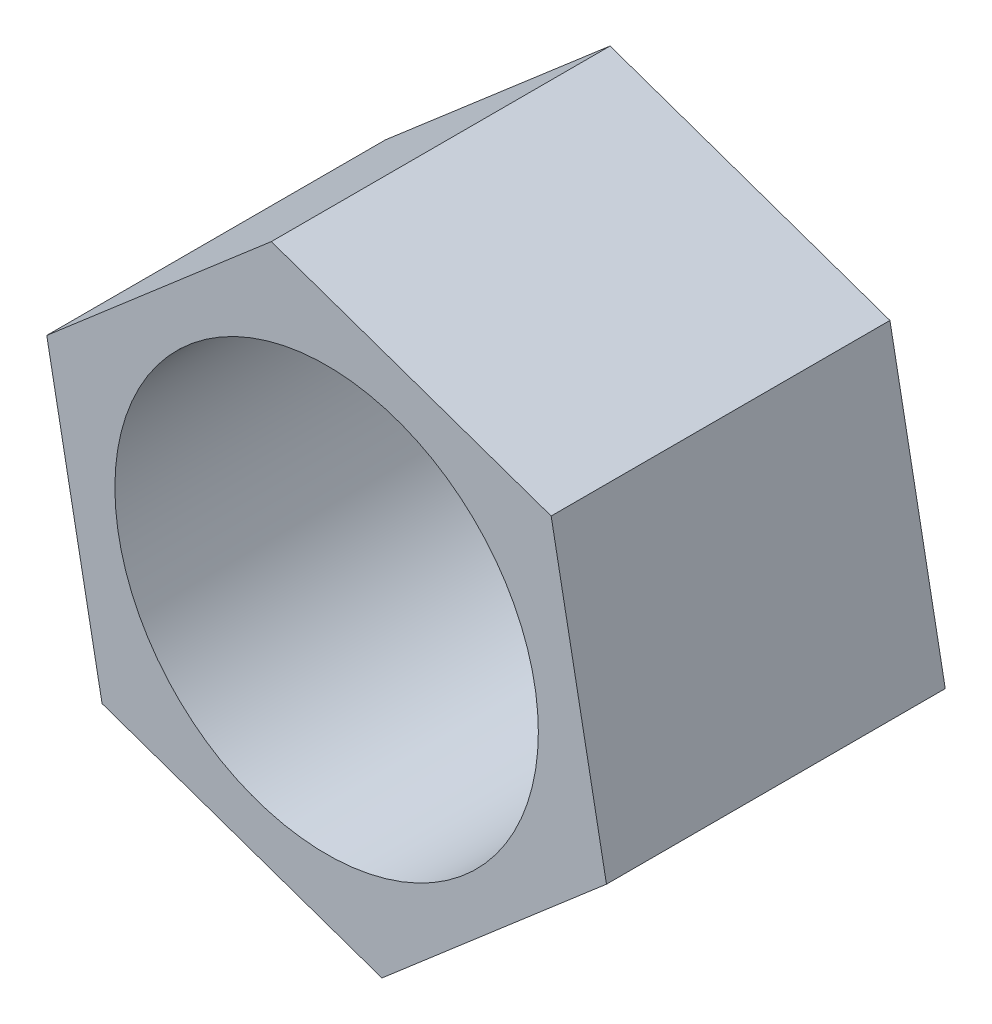
SolidWorks part; units mm, degrees
ref_plane "Front Plane" through (0, 0, 0) normal (0, 0, 1) x (1, 0, 0)
ref_plane "Top Plane" through (0, 0, 0) normal (0, 1, 0) x (1, 0, 0)
ref_plane "Right Plane" through (0, 0, 0) normal (1, 0, 0) x (0, 0, -1)
sketch "Sketch1" plane through (0, 0, 0) normal (0, 0, 1) x (1, 0, 0)
  line L1 (6.7346, 5.8032) -> (-1.6584, 8.7339)
  line L2 (-1.6584, 8.7339) -> (-8.393, 2.9307)
  line L3 (-8.393, 2.9307) -> (-6.7346, -5.8032)
  line L4 (-6.7346, -5.8032) -> (1.6584, -8.7339)
  line L5 (1.6584, -8.7339) -> (8.393, -2.9307)
  line L6 (8.393, -2.9307) -> (6.7346, 5.8032)
  circle A0 centre (0, 0) radius 7.699 construction
  circle A1 centre (0, 0) radius 6.35
  dimension "D1" = 12.7
  dimension "D2" = 17.78
extrude "Boss-Extrude1" add sketch "Sketch1" along normal blind 10.16
scale "Scale1" bodies to scale 101 scale about origin uniform scaling yes scale factor 2
